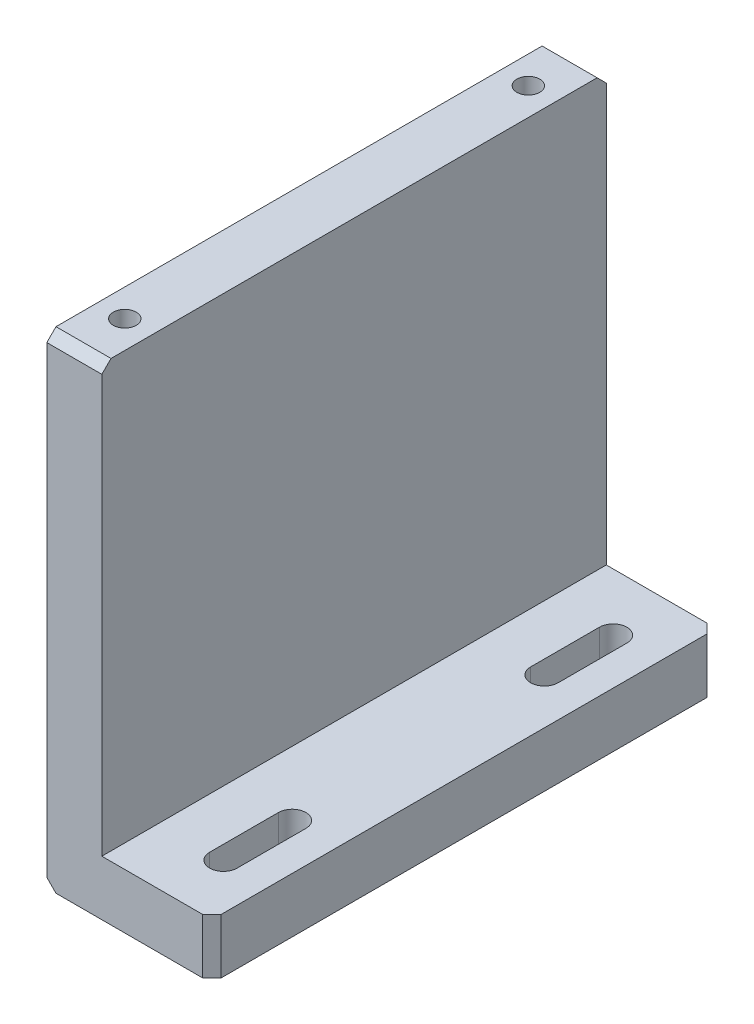
from build123d import *

# Parameters (mm, degrees)
BOSS_EXTRUDE1_DEPTH   = 110
CHAMFER1_SIZE         = 2
CUT_EXTRUDE1_DEPTH    = 150.127637408
M6_TAPPED_HOLE1_D     = 5
M6_TAPPED_HOLE1_DEPTH = 10.497848452
M6_TAPPED_HOLE1_TIP   = 1.502151548


with BuildPart() as part:
    # Sketch1 → Boss-Extrude1 (new body)
    with BuildSketch(Plane.XY):
        Polygon((-38.601194786, 51.777777778), (-38.601194786, -53.222222222), (-2.601194786, -53.222222222), (-2.601194786, -41.222222222), (-26.601194786, -41.222222222), (-26.601194786, 51.777777778), align=None)
    extrude(amount=BOSS_EXTRUDE1_DEPTH)

    # Chamfer1
    chamfer1_edges = [part.edges().sort_by_distance(p)[0] for p in [
        (-38.601194786, -53.222222222, 55),
        (-2.601194786, -47.222222222, 110),
        (-32.601194786, 51.777777778, 110),
        (-2.601194786, -47.222222222, 0),
        (-32.601194786, 51.777777778, 0),
    ]]
    chamfer(chamfer1_edges, length=CHAMFER1_SIZE)

    # Sketch2 → Cut-Extrude1 (cut, through all)
    with BuildSketch(Plane(origin=(0, -41.222222222, 0), x_dir=(1, 0, 0), z_dir=(0, 1, 0))):
        with BuildLine():
            Line((-15.601194786, -97.5), (-15.601194786, -82.5))
            ThreePointArc((-15.601194786, -82.5), (-12.601194786, -79.5), (-9.601194786, -82.5))
            Line((-9.601194786, -82.5), (-9.601194786, -97.5))
            ThreePointArc((-9.601194786, -97.5), (-12.601194786, -100.5), (-15.601194786, -97.5))
        make_face()
        with BuildLine():
            Line((-15.601194786, -12.5), (-15.601194786, -27.5))
            ThreePointArc((-15.601194786, -27.5), (-12.601194786, -30.5), (-9.601194786, -27.5))
            Line((-9.601194786, -27.5), (-9.601194786, -12.5))
            ThreePointArc((-9.601194786, -12.5), (-12.601194786, -9.5), (-15.601194786, -12.5))
        make_face()
    extrude(amount=-CUT_EXTRUDE1_DEPTH, mode=Mode.SUBTRACT)

    # M6 Tapped Hole1
    with Locations(Plane(origin=(0, 51.777777778, 0), x_dir=(1, 0, 0), z_dir=(0, 1, 0))):
        with Locations((-32.601194786, -99), (-32.601194786, -11)):
            Hole(M6_TAPPED_HOLE1_D / 2, depth=M6_TAPPED_HOLE1_DEPTH)
            with Locations((0, 0, -(M6_TAPPED_HOLE1_DEPTH + M6_TAPPED_HOLE1_TIP / 2))):  # 118° drill point
                Cone(0, M6_TAPPED_HOLE1_D / 2, M6_TAPPED_HOLE1_TIP, mode=Mode.SUBTRACT)


solid = part.part
